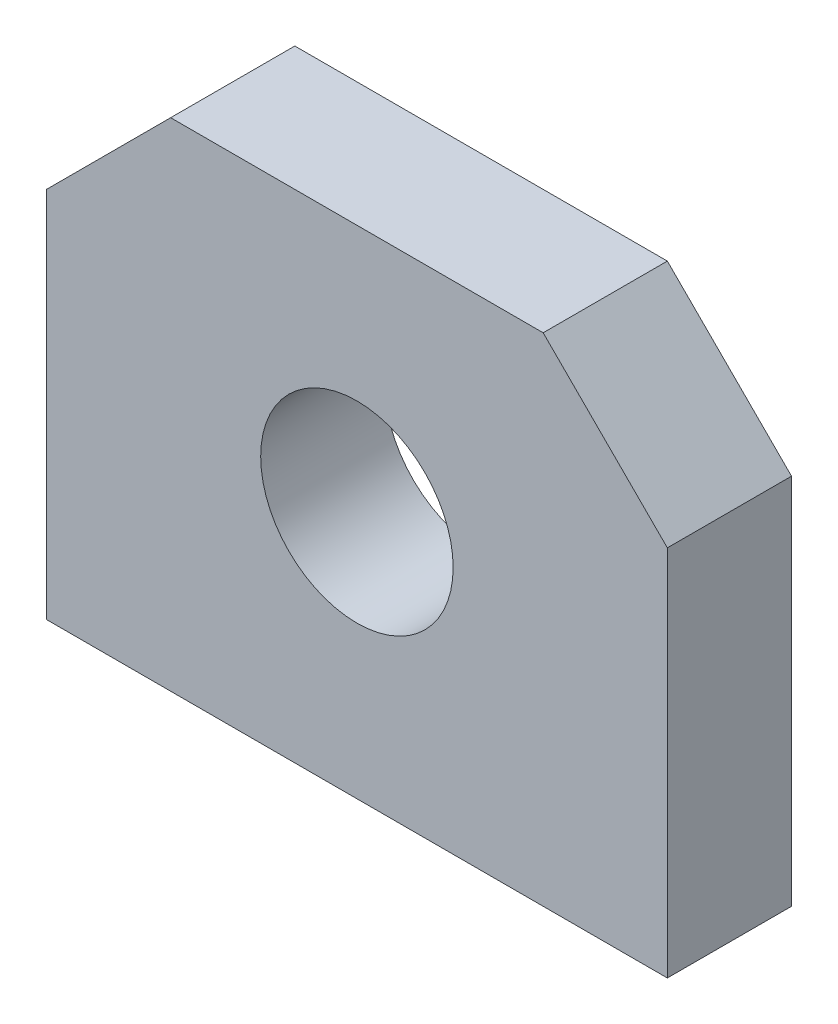
SolidWorks part; units mm, degrees
material "1023 碳钢板 (SS)"
ref_plane "Front Plane" through (0, 0, 0) normal (0, 0, 1) x (1, 0, 0)
ref_plane "Top Plane" through (0, 0, 0) normal (0, 1, 0) x (1, 0, 0)
ref_plane "Right Plane" through (0, 0, 0) normal (1, 0, 0) x (0, 0, -1)
sketch "Sketch1" plane through (0, 0, 0) normal (0, 0, 1) x (1, 0, 0)
  line L1 (25, 20) -> (-25, 20)
  line L2 (25, 20) -> (25, -20)
  line L3 (25, -20) -> (-25, -20)
  line L4 (-25, 20) -> (-25, -20)
  line L5 (25, 20) -> (-25, -20) construction
  line L6 (25, -20) -> (-25, 20) construction
  point P0 (0, 0)
  dimension "D1" = 50
  dimension "D2" = 40
extrude "Boss-Extrude1" add sketch "Sketch1" along normal blind 10 contours L2 L1 L4 L3
chamfer "Chamfer1" distance 10 angle 45 2 edges at (-25, 20, 5) (25, 20, 5)
sketch "Sketch2" plane through (0, 0, 0) normal (0, 0, -1) x (-1, 0, 0)
  line L0 (-15, 20) -> (15, 20) construction
  circle A0 centre (0, 0) radius 8.5282
  dimension "D1" = 20
hole_wizard "M18 Tapped Hole1" positions "Sketch3" profile "Sketch4" tap size "M18" standard "ISO"
sketch "Sketch3" plane through (0, 0, 0) normal (0, 0, -1) x (-1, 0, 0)
  point P0 (0, 0)
sketch "Sketch4" plane through (0, 0, 0) normal (1, 0, 0) x (0, 1, 0)
  line L0 (0, 0) -> (0, 48.1567)
  line L1 (0, 48.1567) -> (7.75, 43.5)
  line L2 (7.75, 43.5) -> (7.75, 0)
  line L5 (7.75, 0) -> (0, 0)
  line L10 (0, 48.1567) -> (-7.75, 43.5) construction
  line L11 (0, -6.35) -> (0, 107.95) construction
  dimension "螺纹孔钻头直径" = 15.5
  dimension "螺纹孔钻头深度" = 43.5
  dimension "导头角度" = 118
cosmetic thread "Hole Thread Line1" parameters "D1"=36, "D2"=18
